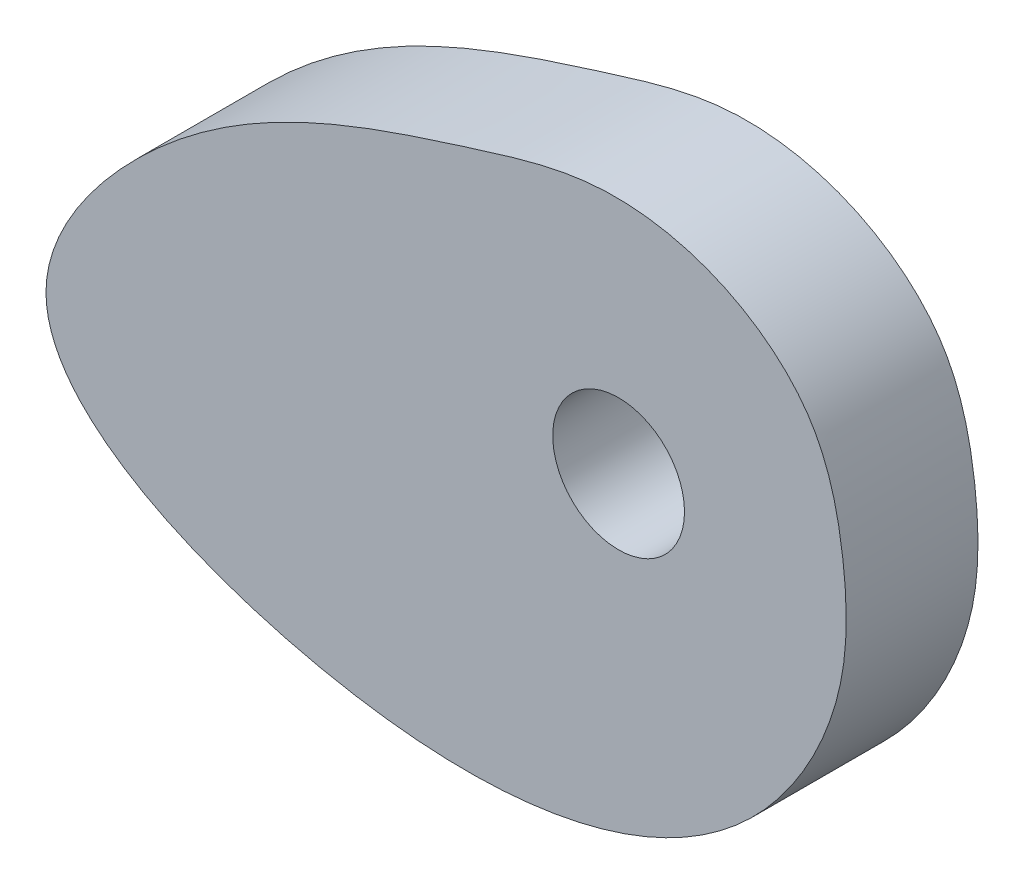
SolidWorks part; units mm, degrees
material "PBT general purpose"
ref_plane "Front Plane" through (0, 0, 0) normal (0, 0, 1) x (1, 0, 0)
ref_plane "Top Plane" through (0, 0, 0) normal (0, 1, 0) x (1, 0, 0)
ref_plane "Right Plane" through (0, 0, 0) normal (1, 0, 0) x (0, 0, -1)
sketch "Sketch1" plane through (0, 0, 0) normal (0, 0, 1) x (1, 0, 0)
  circle A0 centre (0, 0) radius 5
  spline S0 degree 3 poles (17.5152, -6.0908) (17.2451, 3.1878) (15.3767, 11.266) (7.9996, 17.1779) (-1.4795, 18.8085) (-16.4145, 14.213) (-32.4202, 9.0139) (-50.2696, -14.1083) (-17.2347, -28.8144) (9.0412, -23.6347) (17.5152, -6.0908) (17.2451, 3.1878) (15.3767, 11.266) knots -0.340872 -0.123334 -0.046055 0 0.050621 0.103696 0.166927 0.223626 0.393033 0.496899 0.659128 0.876666 0.953945 1 1.050621 1.103696 1.166927 only from (17.0125, 2.9575) to (17.0125, 2.9575)
extrude "Boss-Extrude1" add sketch "Sketch1" along normal blind 10
